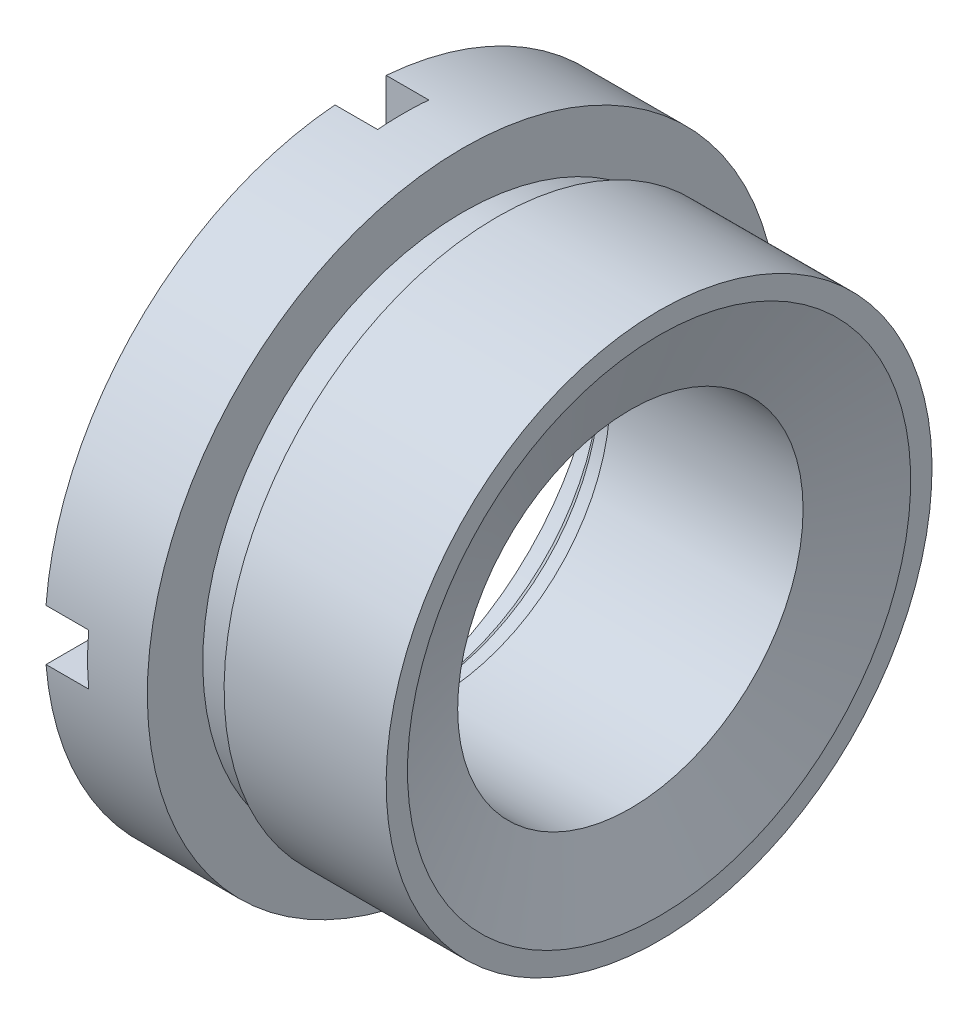
from build123d import *

# Parameters (mm, degrees)
CUT_EXTRUDE1_DEPTH = 5
CIRPATTERN1_COUNT  = 4


with BuildPart() as part:
    # Sketch1 → Revolve1 (revolve)
    with BuildSketch(Plane.XY):
        Polygon((-3.366724667, 20.25), (0, 29.5), (0, 32), (-19, 32), (-19, 30.5), (-23, 30.5), (-23, 32), (-23, 37), (-35, 37), (-35, 28), (-29, 28), (-29, 22), (-28, 21), (-26, 21), (-26, 20.25), align=None)
    revolve(axis=Axis((0, 0, 0), (-1, 0, 0)))

    # Sketch2 → Cut-Extrude1 (cut)
    with BuildSketch(Plane.ZY.offset(35)):
        with BuildLine():
            ThreePointArc((3, 36.878177829), (0, 37), (-3, 36.878177829))
            Line((-3, 36.878177829), (-3, 27.838821814))
            ThreePointArc((-3, 27.838821814), (0, 28), (3, 27.838821814))
            Line((3, 27.838821814), (3, 36.878177829))
        make_face()
    cut_extrude1 = extrude(amount=-CUT_EXTRUDE1_DEPTH, mode=Mode.SUBTRACT)

    # CirPattern1: Cut-Extrude1 ×4 about axis
    cirpattern1_axis = Axis((0, 0, 0), (1, 0, 0))
    for i in range(1, CIRPATTERN1_COUNT):
        add(cut_extrude1.rotate(cirpattern1_axis, i * 360 / CIRPATTERN1_COUNT), mode=Mode.SUBTRACT)


solid = part.part
